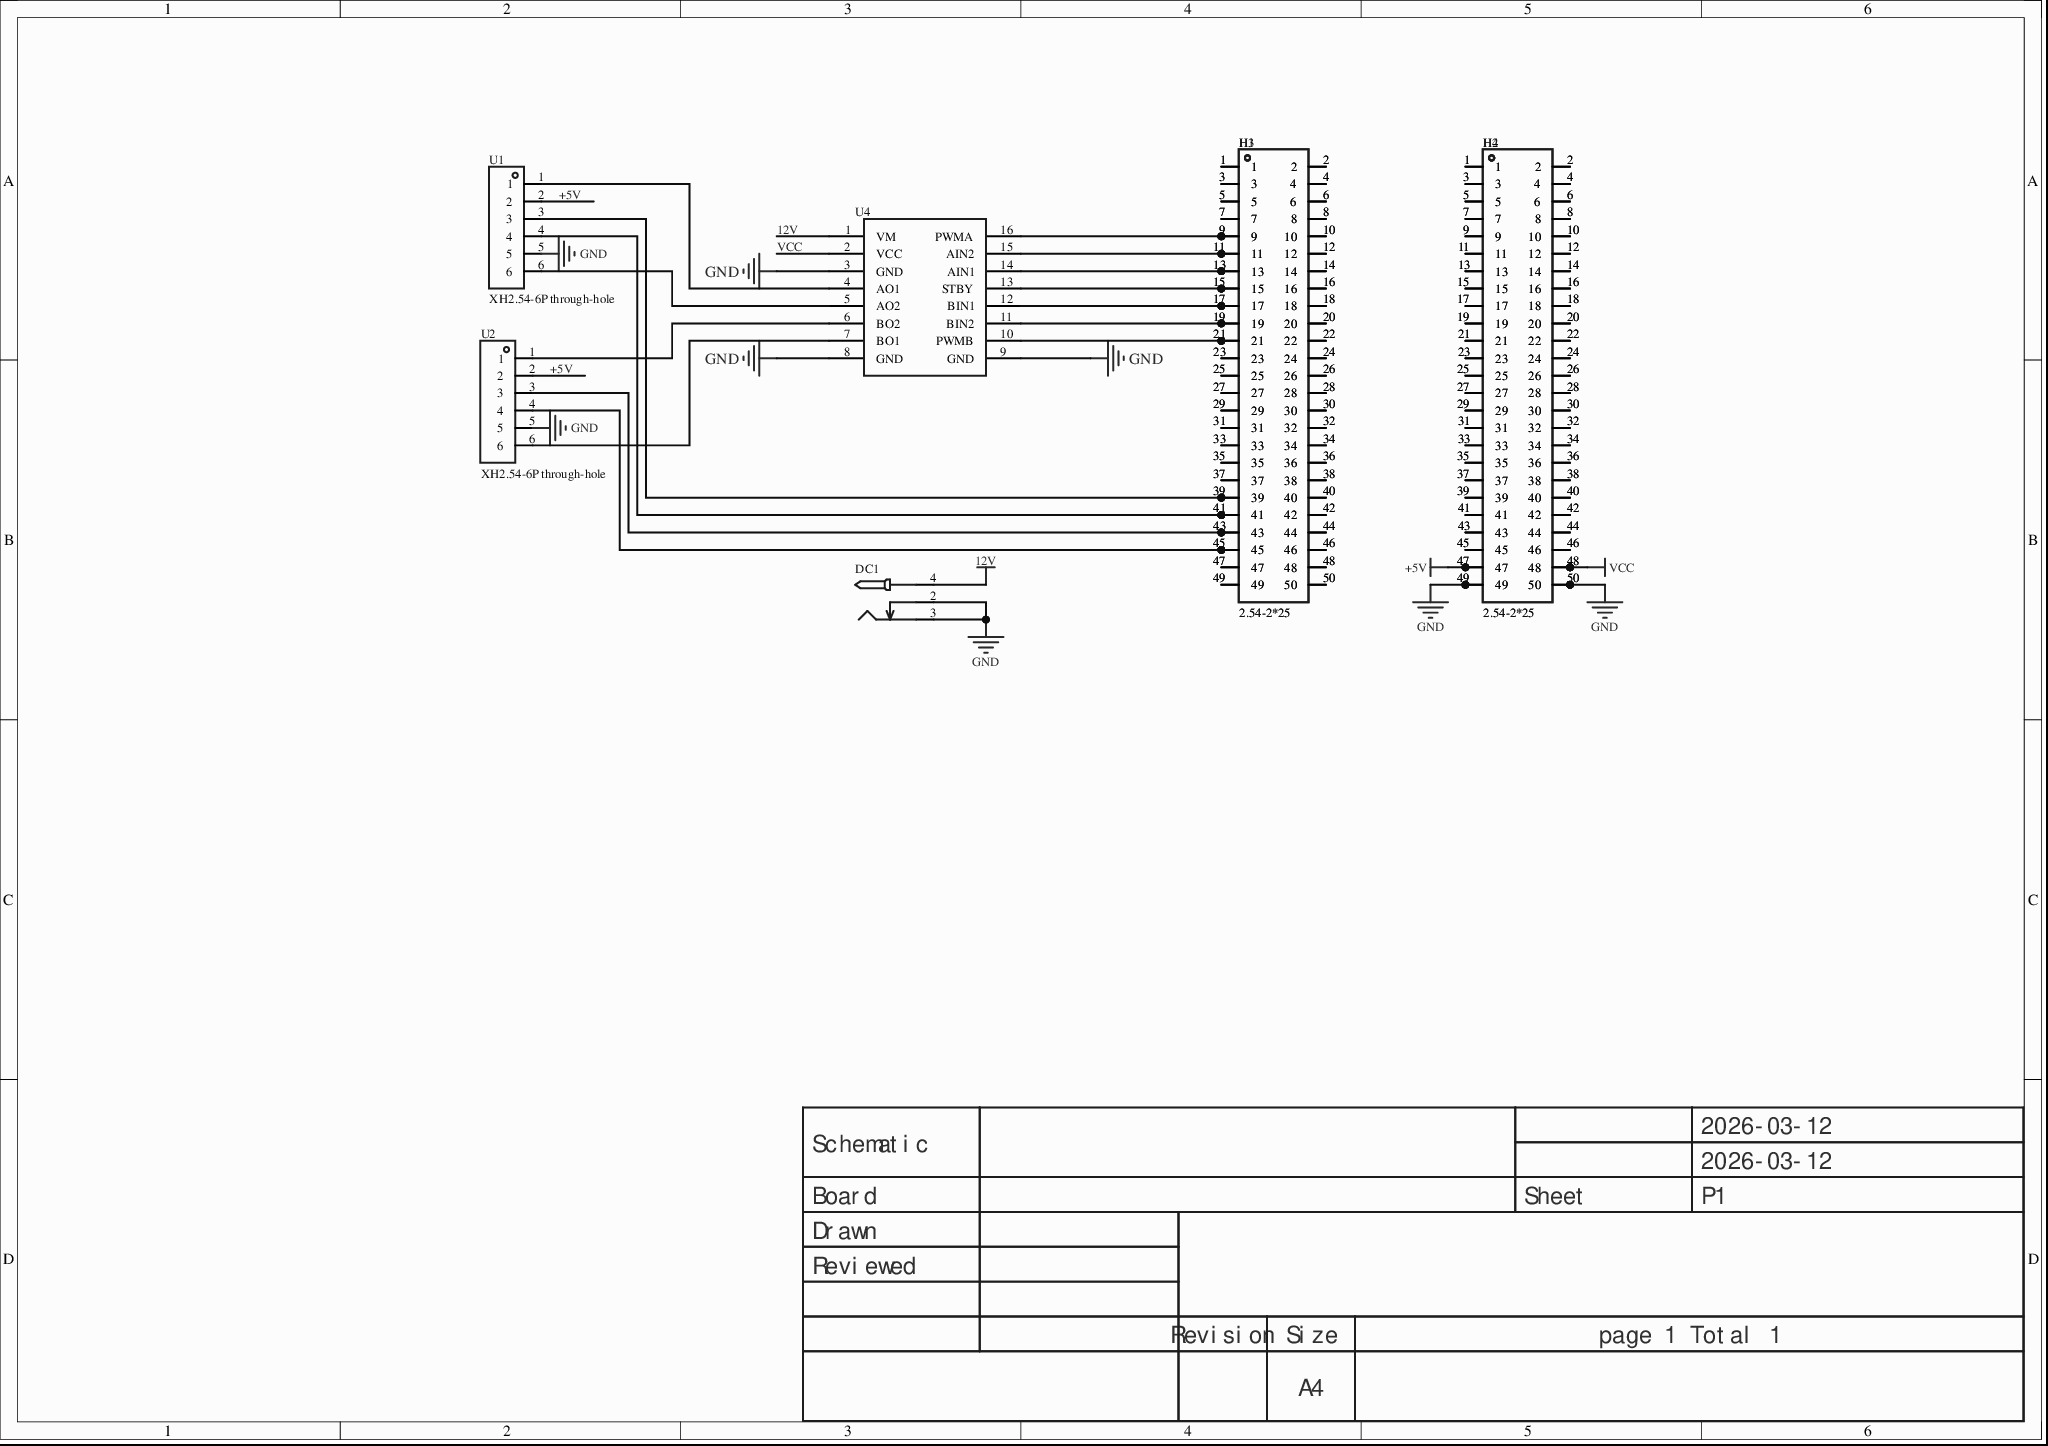
[diagram p0: MISC89017-3.schdoc]
# Altium project MISC89017-2.PrjPcb
1 sheet, 8 parts. Net scope: global (net labels, ports and power ports of the same name join across sheets).
Board file: MISC89017.pcbdoc

## Sheet MISC89017-3.schdoc
size 297 x 209 mm; Version: V1.0; @Project Name: MISC89017; @Update Date: 2026-03-12; @Create Date: 2026-03-12; @Board Name: MISC89017; @Create Time: 23:24:57; @Page Count: 1; @Page No: 1; @Schematic Name: MISC89017; @Update Time: 23:24:57; Size: A4

### Parts
DC1  (no value)  [DC-2.0]
H1  2.54-2*25  [HDR-TH_50P-P2.54-V-F-R2-C25-S2.54-1]
H2  2.54-2*25  [HDR-TH_50P-P2.54-V-F-R2-C25-S2.54-1]
H3  2.54-2*25  [HDR-TH_50P-P2.54-V-F-R2-C25-S2.54-1]
H4  2.54-2*25  [HDR-TH_50P-P2.54-V-F-R2-C25-S2.54-1]
U1  XH2.54-6P through-hole  [CONN-TH_XH2.54-6P]
U2  XH2.54-6P through-hole  [CONN-TH_XH2.54-6P]
U4  (no value)  [tb6612]

### Nets
12V: DC1.4 U4.1(VM)
+5V: H2.47 H4.47 U1.2 U2.2
GND: DC1.2 DC1.3 H2.49 H2.50 H4.49 H4.50 U1.5 U2.5 U4.3(GND) U4.8(GND) U4.9(GND)
VCC: H2.48 H4.48 U4.2(VCC)
NetH1_1: H1.1 H3.1
NetH1_2: H1.2 H3.2
NetH1_3: H1.3 H3.3
NetH1_4: H1.4 H3.4
NetH1_5: H1.5 H3.5
NetH1_6: H1.6 H3.6
NetH1_7: H1.7 H3.7
NetH1_8: H1.8 H3.8
NetH1_9: H1.9 H3.9 U4.16(PWMA)
NetH1_10: H1.10 H3.10
NetH1_11: H1.11 H3.11 U4.15(AIN2)
NetH1_12: H1.12 H3.12
NetH1_13: H1.13 H3.13 U4.14(AIN1)
NetH1_14: H1.14 H3.14
NetH1_15: H1.15 H3.15 U4.13(STBY)
NetH1_16: H1.16 H3.16
NetH1_17: H1.17 H3.17 U4.12(BIN1)
NetH1_18: H1.18 H3.18
NetH1_19: H1.19 H3.19 U4.11(BIN2)
NetH1_20: H1.20 H3.20
NetH1_21: H1.21 H3.21 U4.10(PWMB)
NetH1_22: H1.22 H3.22
NetH1_23: H1.23 H3.23
NetH1_24: H1.24 H3.24
NetH1_25: H1.25 H3.25
NetH1_26: H1.26 H3.26
NetH1_27: H1.27 H3.27
NetH1_28: H1.28 H3.28
NetH1_29: H1.29 H3.29
NetH1_30: H1.30 H3.30
NetH1_31: H1.31 H3.31
NetH1_32: H1.32 H3.32
NetH1_33: H1.33 H3.33
NetH1_34: H1.34 H3.34
NetH1_35: H1.35 H3.35
NetH1_36: H1.36 H3.36
NetH1_37: H1.37 H3.37
NetH1_38: H1.38 H3.38
NetH1_39: H1.39 H3.39 U1.3
NetH1_40: H1.40 H3.40
NetH1_41: H1.41 H3.41 U1.4
NetH1_42: H1.42 H3.42
NetH1_43: H1.43 H3.43 U2.3
NetH1_44: H1.44 H3.44
NetH1_45: H1.45 H3.45 U2.4
NetH1_46: H1.46 H3.46
NetH1_47: H1.47 H3.47
NetH1_48: H1.48 H3.48
NetH1_49: H1.49 H3.49
NetH1_50: H1.50 H3.50
NetH2_1: H2.1 H4.1
NetH2_2: H2.2 H4.2
NetH2_3: H2.3 H4.3
NetH2_4: H2.4 H4.4
NetH2_5: H2.5 H4.5
NetH2_6: H2.6 H4.6
NetH2_7: H2.7 H4.7
NetH2_8: H2.8 H4.8
NetH2_9: H2.9 H4.9
NetH2_10: H2.10 H4.10
NetH2_11: H2.11 H4.11
NetH2_12: H2.12 H4.12
NetH2_13: H2.13 H4.13
NetH2_14: H2.14 H4.14
NetH2_15: H2.15 H4.15
NetH2_16: H2.16 H4.16
NetH2_17: H2.17 H4.17
NetH2_18: H2.18 H4.18
NetH2_19: H2.19 H4.19
NetH2_20: H2.20 H4.20
NetH2_21: H2.21 H4.21
NetH2_22: H2.22 H4.22
NetH2_23: H2.23 H4.23
NetH2_24: H2.24 H4.24
NetH2_25: H2.25 H4.25
NetH2_26: H2.26 H4.26
NetH2_27: H2.27 H4.27
NetH2_28: H2.28 H4.28
NetH2_29: H2.29 H4.29
NetH2_30: H2.30 H4.30
NetH2_31: H2.31 H4.31
NetH2_32: H2.32 H4.32
NetH2_33: H2.33 H4.33
NetH2_34: H2.34 H4.34
NetH2_35: H2.35 H4.35
NetH2_36: H2.36 H4.36
NetH2_37: H2.37 H4.37
NetH2_38: H2.38 H4.38
NetH2_39: H2.39 H4.39
NetH2_40: H2.40 H4.40
NetH2_41: H2.41 H4.41
NetH2_42: H2.42 H4.42
NetH2_43: H2.43 H4.43
NetH2_44: H2.44 H4.44
NetH2_45: H2.45 H4.45
NetH2_46: H2.46 H4.46
NetU1_1: U1.1 U4.4(AO1)
NetU1_6: U1.6 U4.5(AO2)
NetU2_1: U2.1 U4.6(BO2)
NetU2_6: U2.6 U4.7(BO1)

### Notes on the sheet
- 2026-03-12
- Schematic
- Board
- Sheet
- P1
- Drawn
- Reviewed
- Revision
- Size
- A4
- page 1 Total 1

### Library data of the parts
DC1 = DC-005_2.0: Symbol: DC power jack; ConvertToPcb: yes; ModelId: f5f20b8a2308479b936ba3c2698865bb0819f05c4eef4c71ace90d822a990e87; ModelName: DC-IN-TH_DC-5520-1; ModelTransform: 372.05,551.18,582.68,90,0,0,137.8,0,-149.61; Device: DC-005_2.0; AddInBom: yes; Supplier Footprint: 插件; FootprintName: DC-2.0
H1 H2 = 2.54-2*25: 插孔结构:2x25P;间距:2.54mm;行距:2.54mm;圆孔/方孔:方孔;安装方式:直插;排数:双排;总孔位数:50P;额定电流:2.5A;插孔方向:顶部;塑高:8.5mm;触头材质:黄铜;工作温度:-40℃~+105℃;; Manufacturer: ZHOURI(洲日); AddInBom: yes; ModelId: a9958256e3444847b8d486b2c0cfe9f00819f05c4eef4c71ace90d822a990e87; ModelName: HDR2.54-F-LI-2X25P; ModelTransform: 2499.995,200,0,0,0,0,0,0,-118.11; Holes Structure: 2x25P; Pitch: 2.54mm; Circular Hole / Square Hole: Square hole; Number of Positions: 50P; Current Rating: 2.5A; Holes Direction: Top; PIN Length: 3.2mm; Symbol: 2.54-2*25; Device: 2.54-2*25; LCSC Part Name: 2x25P 间距:2.54mm 直插; SupplierPart: C5116487; ManufacturerPart: 2.54-2*25; Supplier Footprint: 插件,P=2.54mm; JLCPCB Part Class: Extended Part; Datasheet: example.com/datasheet/2.54-2*25/5692730.html; Supplier: LCSC; ConvertToPcb: yes; FootprintName: HDR-TH_50P-P2.54-V-F-R2-C25-S2.54-1; Row Spacing: 2.54mm; Mounting Type: Through-hole; Number of Rows: Double row; Insulation Height: 8.5mm; Contact Material: Brass; Operating Temperature: -40℃~+105℃
H3 H4 = 2.54-2*25: 插孔结构:2x25P;间距:2.54mm;行距:2.54mm;圆孔/方孔:方孔;安装方式:直插;排数:双排;总孔位数:50P;额定电流:2.5A;插孔方向:顶部;塑高:8.5mm;触头材质:黄铜;工作温度:-40℃~+105℃;; Manufacturer: ZHOURI(洲日); 3D Model: a9958256e3444847b8d486b2c0cfe9f00819f05c4eef4c71ace90d822a990e87; 3D Model Transform: 2499.995,200,0,0,0,0,0,0,-118.11; Holes Structure: 2x25P; Pitch: 2.54mm; Circular Hole / Square Hole: Square hole; Number of Positions: 50P; Current Rating: 2.5A; Holes Direction: Top; PIN Length: 3.2mm; AddInBom: yes; ModelName: HDR2.54-F-LI-2X25P; Symbol: 2.54-2*25; Device: 2.54-2*25; LCSC Part Name: 2x25P 间距:2.54mm 直插; Supplier Part: C5116487; Manufacturer Part: 2.54-2*25; Supplier Footprint: 插件,P=2.54mm; JLCPCB Part Class: Extended Part; Datasheet: example.com/datasheet/2.54-2*25/5692730.html; Supplier: LCSC; Row Spacing: 2.54mm; Mounting Type: Through-hole; Number of Rows: Double row; Insulation Height: 8.5mm; Contact Material: Brass; Operating Temperature: -40℃~+105℃; ConvertToPcb: yes; FootprintName: HDR-TH_50P-P2.54-V-F-R2-C25-S2.54-1
U1 U2 = XH2.54-6P 直插: AddInBom: yes; ModelId: a7224aacb0dc4305a7392217f7fd8fe20819f05c4eef4c71ace90d822a990e87; ModelTransform: 688.975,224.409,0,0,0,0,-0.001,-17.719,-118.11; Symbol: XH2.54-6P; Device: XH2.54-6P through-hole; LCSC Part Name: XH2.54-6P 直插; SupplierPart: C9900000754; ManufacturerPart: XH2.54-6P 直插; Supplier Footprint: TH-6_5.8X17.5X2.54P; JLCPCB Part Class: Extended Part; Supplier: LCSC; ConvertToPcb: yes; FootprintName: CONN-TH_XH2.54-6P; ModelName: CONN-TH_XH2.54-6P
U4 = tb6612: AddInBom: yes; Symbol: tb6612; Device: tb6612; JLCPCB Part Class: Extended library; ConvertToPcb: yes; FootprintName: tb6612